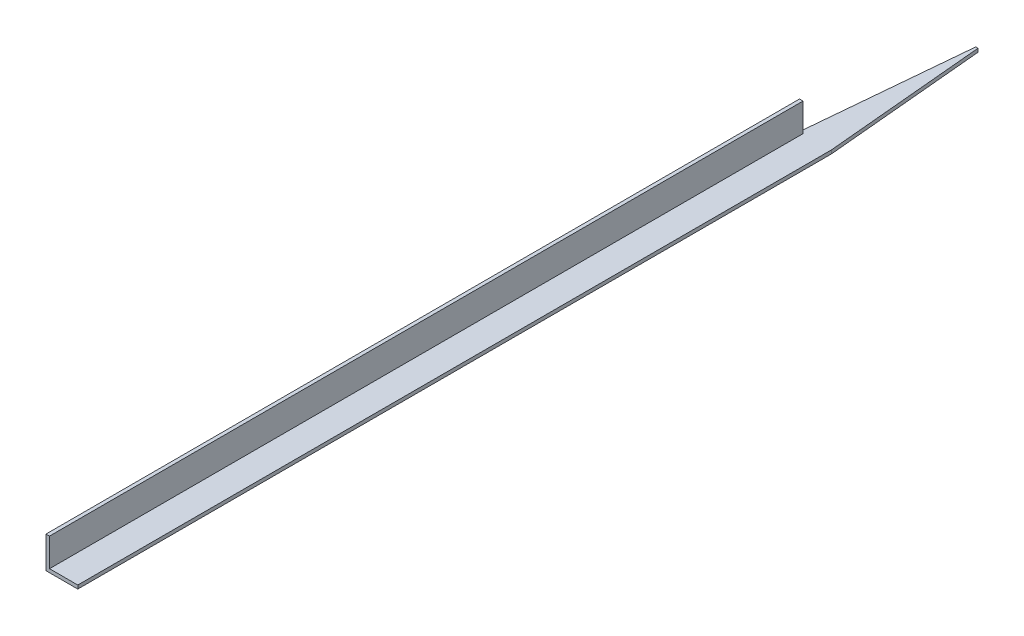
from build123d import *

# Parameters (mm, degrees)
EXTRUDE1_DEPTH = 1295.4
EXTRUDE2_DEPTH = 1297.627083248
SKETCH5_W      = 54.662840746
SKETCH5_H      = 40
EXTRUDE3_DEPTH = 1297.759359805


with BuildPart() as part:
    # Sketch1 → Extrude1 (new body)
    with BuildSketch(Plane.XY):
        Polygon((-11.005397301, 1.140254873), (-11.005397301, -43.859745127), (33.994602699, -43.859745127), (33.994602699, -38.859745127), (-6.005397301, -38.859745127), (-6.005397301, 1.140254873), align=None)
    extrude(amount=EXTRUDE1_DEPTH)

    # Sketch2 → Extrude2 (cut, through all)
    with BuildSketch(Plane.XZ.offset(43.859745127)):
        Polygon((-11.005397301, 0), (9.904602699, 0), (-11.005397301, 228.6), align=None)
        Polygon((33.994602699, 228.6), (13.084602699, 0), (33.994602699, 0), align=None)
    extrude(amount=-EXTRUDE2_DEPTH, mode=Mode.SUBTRACT)

    # Sketch5 → Extrude3 (cut, through all)
    with BuildSketch(Plane(origin=(-6.005397301, 0, 0), x_dir=(0, 0, -1), z_dir=(1, 0, 0))):
        with Locations((-201.268579627, -18.859745127)):
            Rectangle(SKETCH5_W, SKETCH5_H)
    extrude(amount=-EXTRUDE3_DEPTH, mode=Mode.SUBTRACT)


solid = part.part
